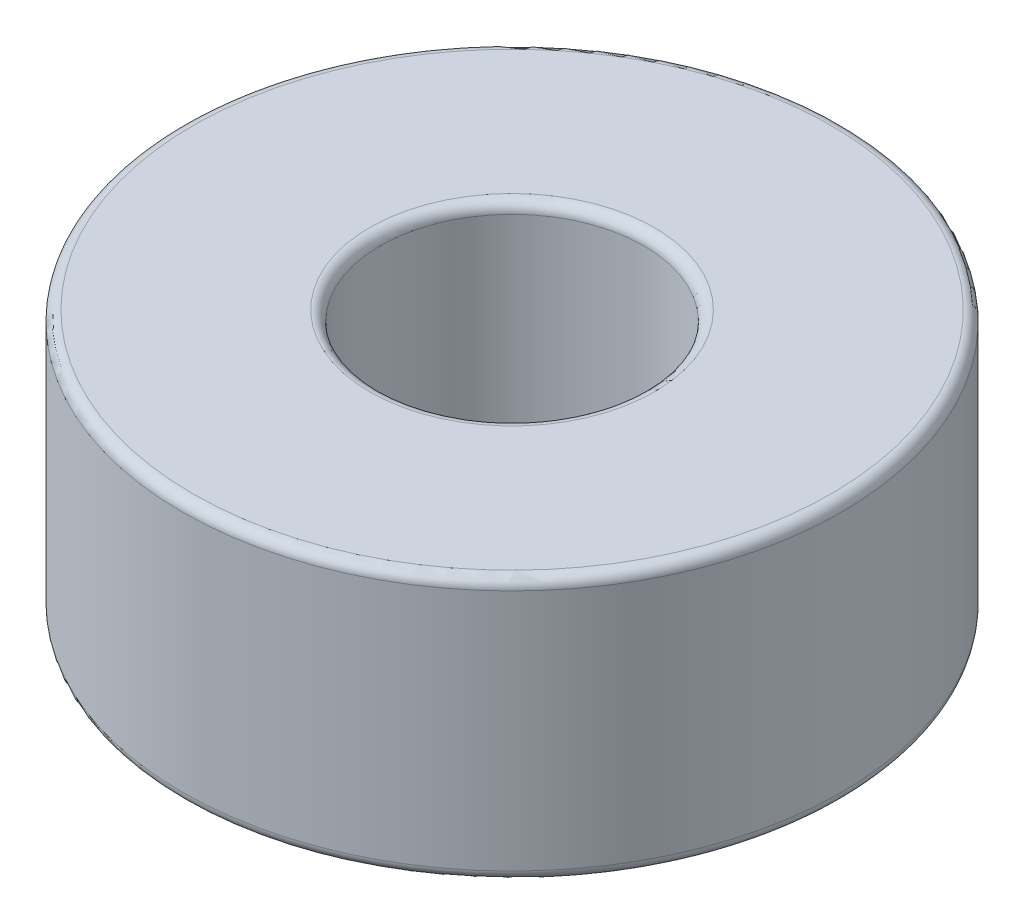
SolidWorks part; units mm, degrees
material "镀铬不锈钢"
ref_plane "前视基准面" through (0, 0, 0) normal (0, 0, 1) x (1, 0, 0)
ref_plane "上视基准面" through (0, 0, 0) normal (0, 1, 0) x (1, 0, 0)
ref_plane "右视基准面" through (0, 0, 0) normal (1, 0, 0) x (0, 0, -1)
sketch "草图1" plane through (0, 0, 0) normal (0, 1, 0) x (1, 0, 0)
  circle A0 centre (0, 0) radius 1
  circle A1 centre (0, 0) radius 2.5
  dimension "D1" = 2
  dimension "D2" = 5
extrude "凸台-拉伸1" add sketch "草图1" along normal blind 2
fillet "R0.08 圆角1" radius 0.08 4 edges at (0, 0, 2.5) (0, 2, 2.5) (0, 0, 1) (0, 2, 1)
